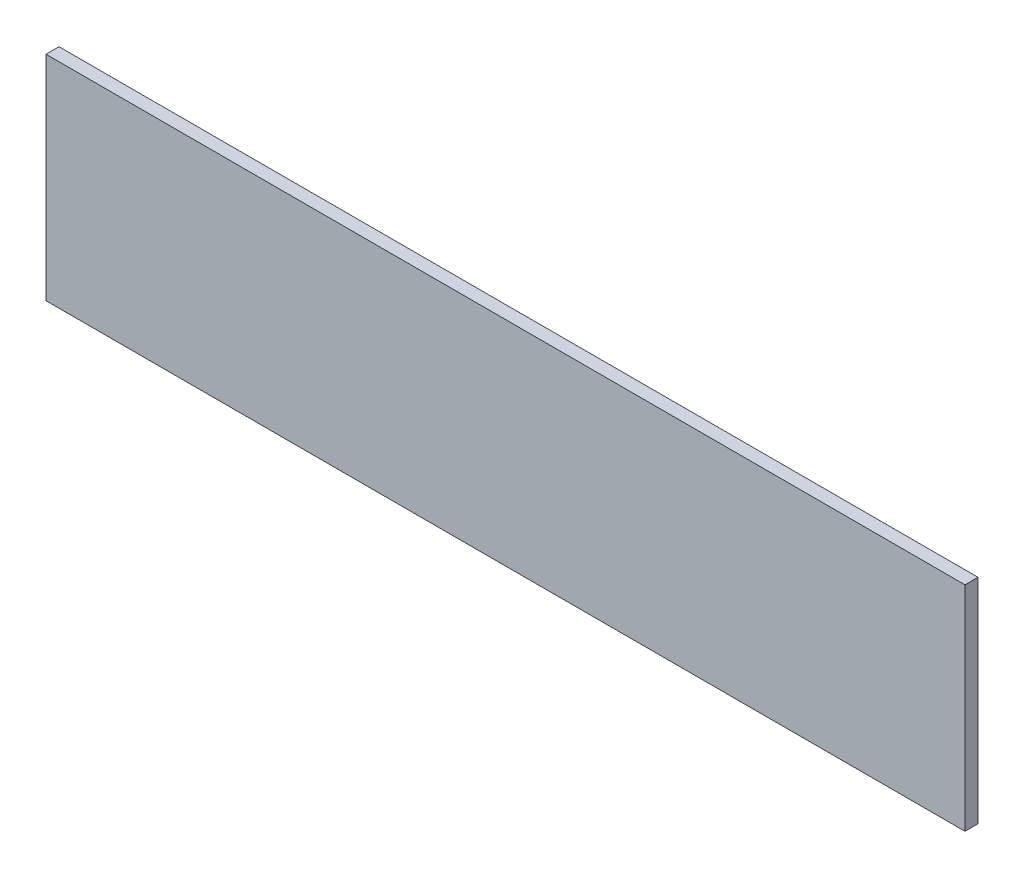
SolidWorks part; units mm, degrees
material "Q235"
ref_plane "Front Plane" through (0, 0, 0) normal (0, 0, 1) x (1, 0, 0)
ref_plane "Top Plane" through (0, 0, 0) normal (0, 1, 0) x (1, 0, 0)
ref_plane "Right Plane" through (0, 0, 0) normal (1, 0, 0) x (0, 0, -1)
sketch "Sketch1" plane through (0, 0, 0) normal (0, 0, 1) x (1, 0, 0)
  line L1 (0, 0) -> (2118, 0)
  line L2 (0, 0) -> (0, 492)
  line L3 (0, 492) -> (2118, 492)
  line L4 (2118, 0) -> (2118, 492)
  dimension "D1" = 2118
  dimension "D2" = 492
extrude "Boss-Extrude1" add sketch "Sketch1" along normal blind 30
